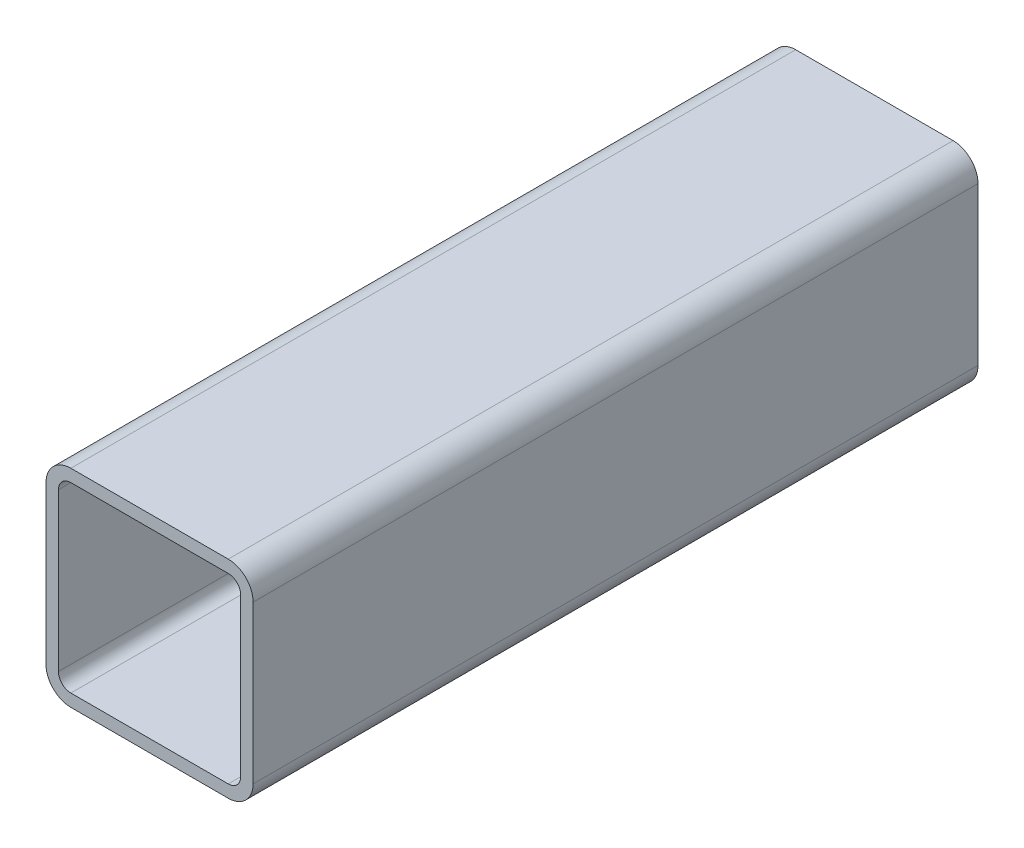
from build123d import *

# Parameters (mm, degrees)
GB_6728_1986_050_X_50_X_3_1_DEPTH = 175


with BuildPart() as part:
    # Sketch1 → Gb／6728-1986方形空心型钢 050 X 50 X 3(1) (new body)
    with BuildSketch(Plane.YX.offset(-87.5)):
        with BuildLine():
            Line((-19, -25), (19, -25))
            ThreePointArc((19, -25), (23.242640687, -23.242640687), (25, -19))
            Line((25, -19), (25, 19))
            ThreePointArc((25, 19), (23.242640687, 23.242640687), (19, 25))
            Line((19, 25), (-19, 25))
            ThreePointArc((-19, 25), (-23.242640687, 23.242640687), (-25, 19))
            Line((-25, 19), (-25, -19))
            ThreePointArc((-25, -19), (-23.242640687, -23.242640687), (-19, -25))
        make_face()
        with BuildLine():
            Line((-19, -22), (19, -22))
            ThreePointArc((19, -22), (21.121320344, -21.121320344), (22, -19))
            Line((22, -19), (22, 19))
            ThreePointArc((22, 19), (21.121320344, 21.121320344), (19, 22))
            Line((19, 22), (-19, 22))
            ThreePointArc((-19, 22), (-21.121320344, 21.121320344), (-22, 19))
            Line((-22, 19), (-22, -19))
            ThreePointArc((-22, -19), (-21.121320344, -21.121320344), (-19, -22))
        make_face(mode=Mode.SUBTRACT)
    extrude(amount=GB_6728_1986_050_X_50_X_3_1_DEPTH)


solid = part.part
